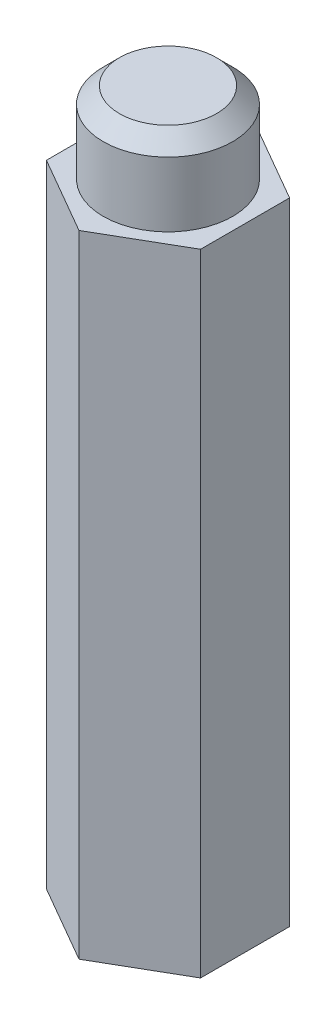
from build123d import *

# Parameters (mm, degrees)
BOSS_EXTRUDE1_DEPTH = 19.5
SKETCH3_R           = 4
BOSS_EXTRUDE2_DEPTH = 5
CHAMFER1_SIZE       = 1


with BuildPart() as part:
    # Sketch1 → Boss-Extrude1 (new, symmetric)
    with BuildSketch(Plane(origin=(0, 0, 0), x_dir=(1, 0, 0), z_dir=(0, 1, 0))):
        Polygon((0, 5.5), (-4.763139721, 2.75), (-4.763139721, -2.75), (0, -5.5), (4.763139721, -2.75), (4.763139721, 2.75), align=None)
    extrude(amount=BOSS_EXTRUDE1_DEPTH, both=True)

    # Sketch3 → Boss-Extrude2 (add)
    with BuildSketch(Plane(origin=(0, 19.5, 0), x_dir=(1, 0, 0), z_dir=(0, 1, 0))):
        with Locations(Location((0, 0, 0), (0, 0, 270))):
            Circle(SKETCH3_R)
    extrude(amount=BOSS_EXTRUDE2_DEPTH)

    # Chamfer1
    chamfer1_edges = [part.edges().sort_by_distance(p)[0] for p in [
        (0, 24.5, -4),
    ]]
    chamfer(chamfer1_edges, length=CHAMFER1_SIZE)

    # Sketch6 → M6x1.0 Tapped Hole2 (revolve, cut)
    with BuildSketch(Plane(origin=(-4.548e-06, -19.5, 2.5825e-05), x_dir=(0, 0, -1), z_dir=(1, 0, 0))):
        Polygon((0, 0), (0, 9.502151548), (2.5, 8), (2.5, 0), align=None)
    revolve(axis=Axis((-4.548e-06, -25.85, 2.5825e-05), (0, 1, 0)), mode=Mode.SUBTRACT)


solid = part.part
